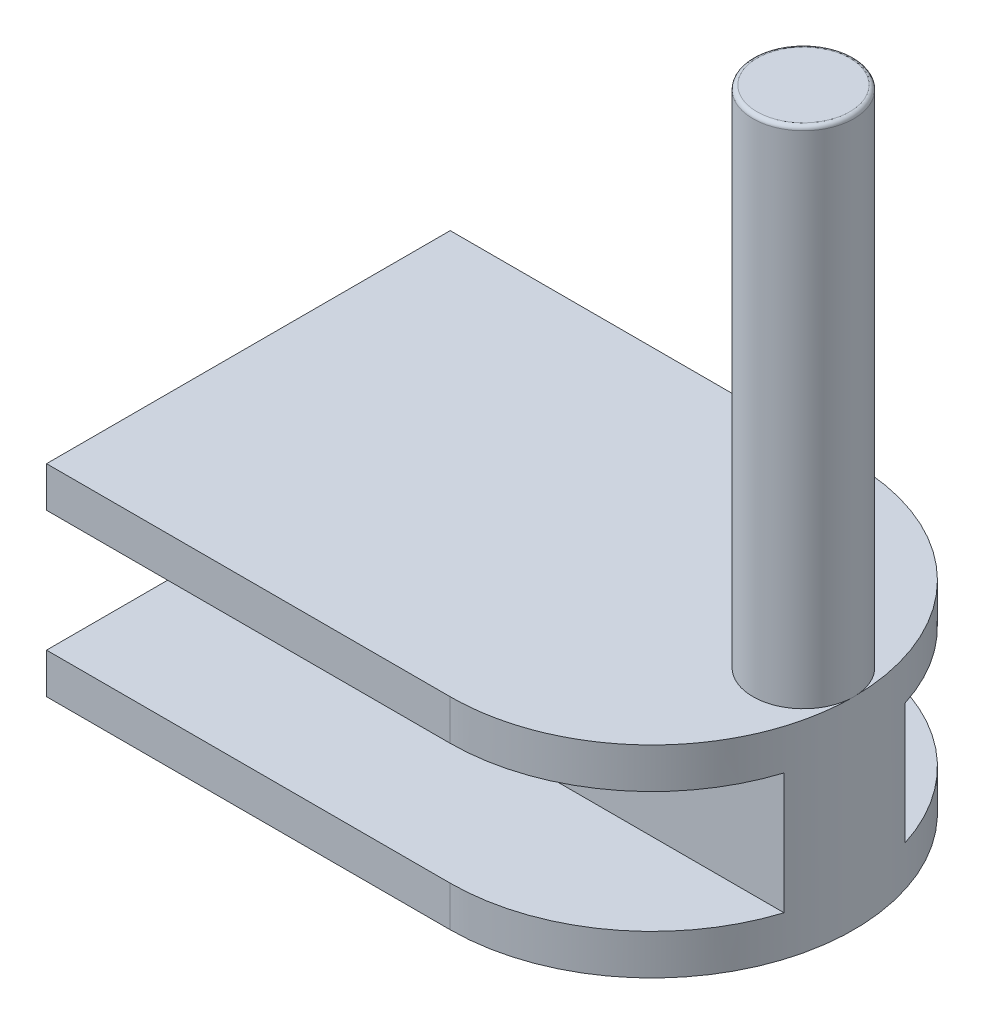
from build123d import *

# Parameters (mm, degrees)
SKETCH1_W           = 30
SKETCH1_H           = 20
BOSS_EXTRUDE1_DEPTH = 10
SKETCH2_W           = 7
SKETCH2_H           = 6
CUT_EXTRUDE1_DEPTH  = 38.416573868
CUT_EXTRUDE2_DEPTH  = 38.416573868
SKETCH4_R           = 2.5
BOSS_EXTRUDE2_DEPTH = 25
FILLET1_R           = 0.2


with BuildPart() as part:
    # Sketch1 → Boss-Extrude1 (new body)
    with BuildSketch(Plane(origin=(0, 0, 0), x_dir=(1, 0, 0), z_dir=(0, 1, 0))):
        with Locations((15, 10)):
            Rectangle(SKETCH1_W, SKETCH1_H)
    extrude(amount=BOSS_EXTRUDE1_DEPTH)

    # Sketch2 → Cut-Extrude1 (cut, through all)
    with BuildSketch(Plane.ZY):
        with Locations((-16.5, 5)):
            Rectangle(SKETCH2_W, SKETCH2_H)
        with Locations((-3.5, 5)):
            Rectangle(SKETCH2_W, SKETCH2_H)
    extrude(amount=-CUT_EXTRUDE1_DEPTH, mode=Mode.SUBTRACT)

    # Sketch3 → Cut-Extrude2 (cut, through all)
    with BuildSketch(Plane(origin=(0, 10, 0), x_dir=(1, 0, 0), z_dir=(0, 1, 0))):
        with BuildLine():
            Line((30, 0), (30, 10))
            ThreePointArc((30, 10), (27.071067812, 2.928932188), (20, 0))
            Line((20, 0), (30, 0))
        make_face()
        with BuildLine():
            Line((30, 10), (30, 20))
            Line((30, 20), (20, 20))
            ThreePointArc((20, 20), (27.071067812, 17.071067812), (30, 10))
        make_face()
    extrude(amount=-CUT_EXTRUDE2_DEPTH, mode=Mode.SUBTRACT)

    # Sketch4 → Boss-Extrude2 (add)
    with BuildSketch(Plane(origin=(0, 10, 0), x_dir=(1, 0, 0), z_dir=(0, 1, 0))):
        with Locations(Location((27.5, 10, 0), (0, 0, 359.999408267))):
            Circle(SKETCH4_R)
    extrude(amount=BOSS_EXTRUDE2_DEPTH)

    # Fillet1
    fillet1_edges = [part.edges().sort_by_distance(p)[0] for p in [
        (25, 35, -10.000025819),
    ]]
    fillet(fillet1_edges, radius=FILLET1_R)


solid = part.part
